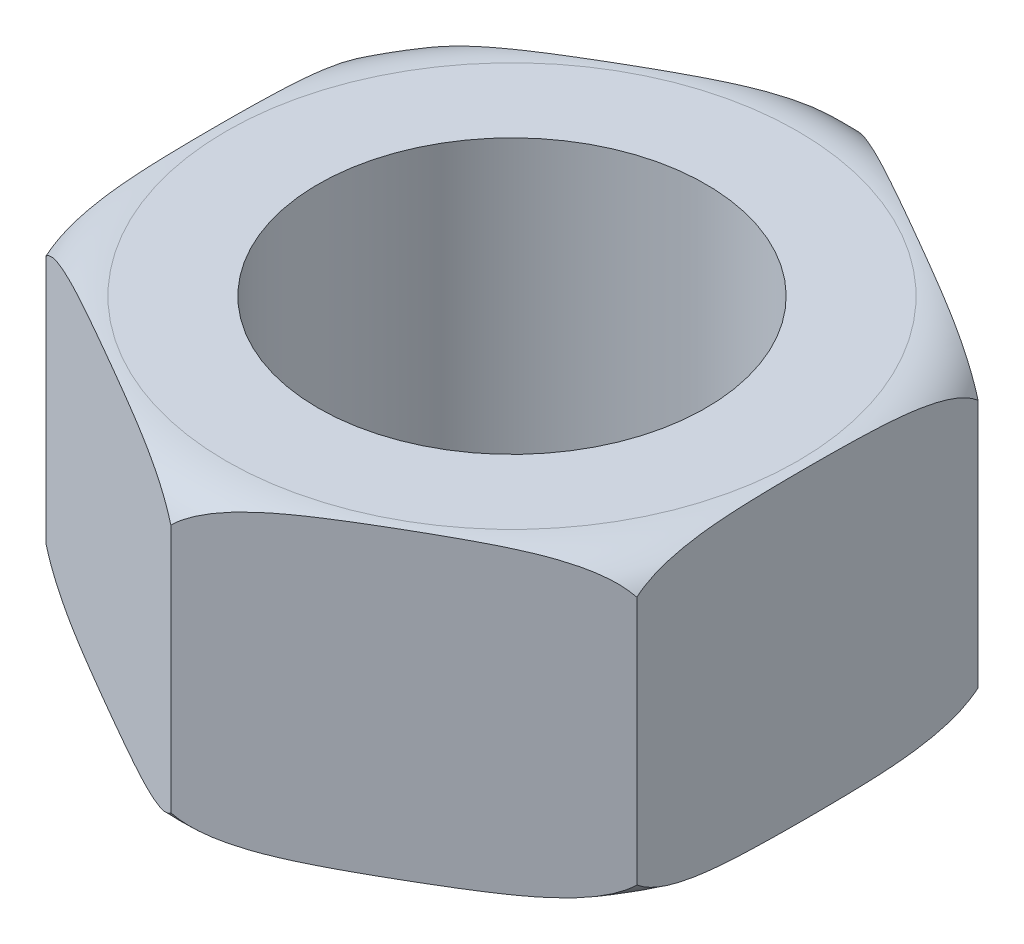
SolidWorks part; units mm, degrees
ref_plane "Front Plane" through (0, 0, 0) normal (0, 0, 1) x (1, 0, 0)
ref_plane "Top Plane" through (0, 0, 0) normal (0, 1, 0) x (1, 0, 0)
ref_plane "Right Plane" through (0, 0, 0) normal (1, 0, 0) x (0, 0, -1)
sketch "Sketch 1" plane through (0, 0, 0) normal (0, 1, 0) x (1, 0, 0)
  line L1 (0, 36.9504) -> (-32, 18.4752)
  line L2 (-32, 18.4752) -> (-32, -18.4752)
  line L3 (-32, -18.4752) -> (0, -36.9504)
  line L4 (0, -36.9504) -> (32, -18.4752)
  line L5 (32, -18.4752) -> (32, 18.4752)
  line L6 (32, 18.4752) -> (0, 36.9504)
  circle A0 centre (0, 0) radius 21
  circle A1 centre (0, 0) radius 32 construction
  dimension "D1" = 42
  dimension "D2" = 64
extrude "Boss-Extrude 1" add sketch "Sketch 1" along normal mid plane 33
sketch "Sketch 2" plane through (0, 0, 0) normal (1, 0, 0) x (0, 0, -1)
  line L0 (0, 20.7202) -> (0, -24.738) construction
  line L1 (-40.7516, 0) -> (40.6368, 0) construction
  line L2 (-36.9504, 16.5) -> (-36.9504, -16.5) construction
  line L3 (-18.4752, 16.5) -> (18.4752, 16.5) construction
  line L4 (-30.9504, 16.5) -> (-36.9504, 16.5)
  line L5 (-36.9504, 16.5) -> (-36.9504, 13.5)
  line L8 (-36.9504, -16.5) -> (-36.9504, -13.5)
  line L9 (-30.9504, -16.5) -> (-36.9504, -16.5)
  spline S0 degree 3 poles (-36.9504, 13.5) (-35.689, 15.629) (-33.3718, 16.5) (-30.9504, 16.5) knots 0 0 0 0 1 1 1 1
  spline S1 degree 3 poles (-36.9504, -13.5) (-35.689, -15.629) (-33.3718, -16.5) (-30.9504, -16.5) knots 0 0 0 0 1 1 1 1
  dimension "D1" = 2
  dimension "D2" = 3
  dimension "D3" = 6
  dimension "D4" = 1
revolve "Cut-Revolve 1" cut sketch "Sketch 2" angle 360 about L0
